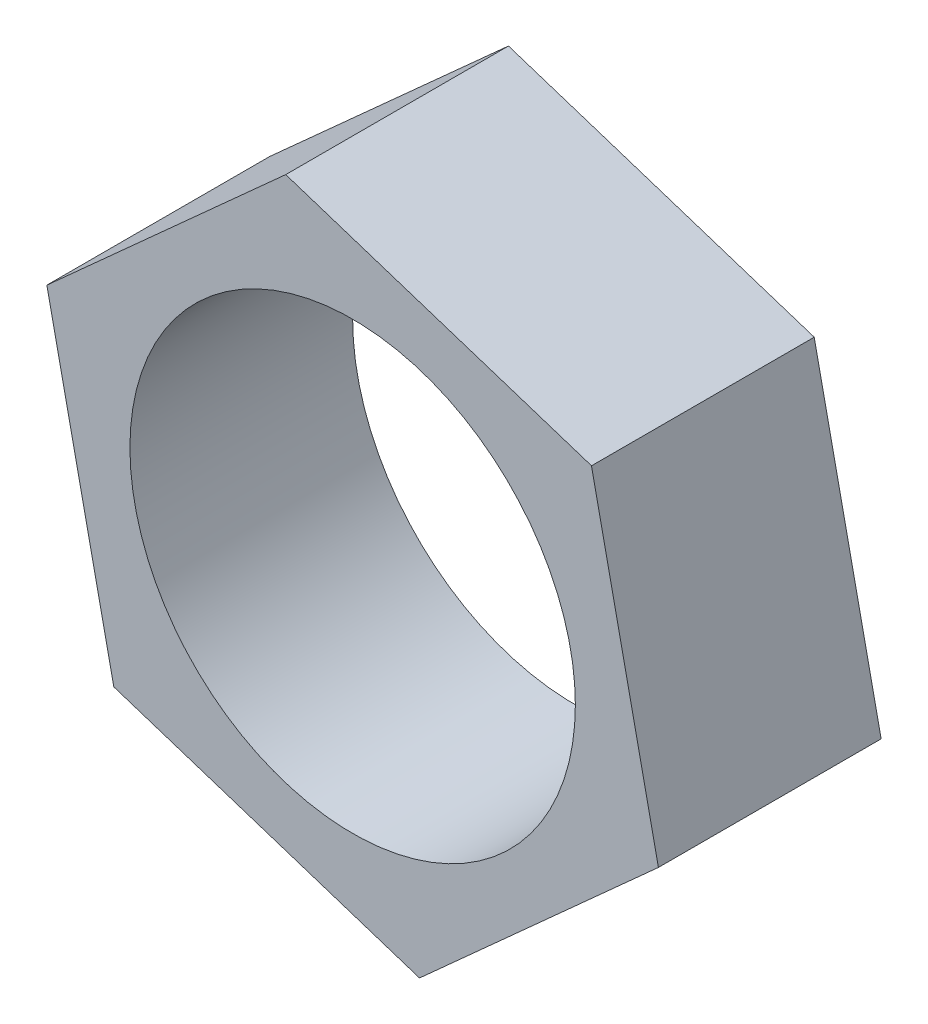
SolidWorks part; units mm, degrees
ref_plane "Front Plane" through (0, 0, 0) normal (0, 0, 1) x (1, 0, 0)
ref_plane "Top Plane" through (0, 0, 0) normal (0, 1, 0) x (1, 0, 0)
ref_plane "Right Plane" through (0, 0, 0) normal (1, 0, 0) x (0, 0, -1)
other "Configuration Table"
sketch "Sketch1" plane through (0, 0, 0) normal (0, 0, 1) x (1, 0, 0)
  line L1 (10.7247, 9.66) -> (-3.0034, 14.1178)
  line L2 (-3.0034, 14.1178) -> (-13.7281, 4.4579)
  line L3 (-13.7281, 4.4579) -> (-10.7247, -9.66)
  line L4 (-10.7247, -9.66) -> (3.0034, -14.1178)
  line L5 (3.0034, -14.1178) -> (13.7281, -4.4579)
  line L6 (13.7281, -4.4579) -> (10.7247, 9.66)
  circle A0 centre (0, 0) radius 12.5 construction
  circle A1 centre (0, 0) radius 10
  dimension "D2" = 20
  dimension "D1" = 25
extrude "Boss-Extrude1" add sketch "Sketch1" along normal blind 10
